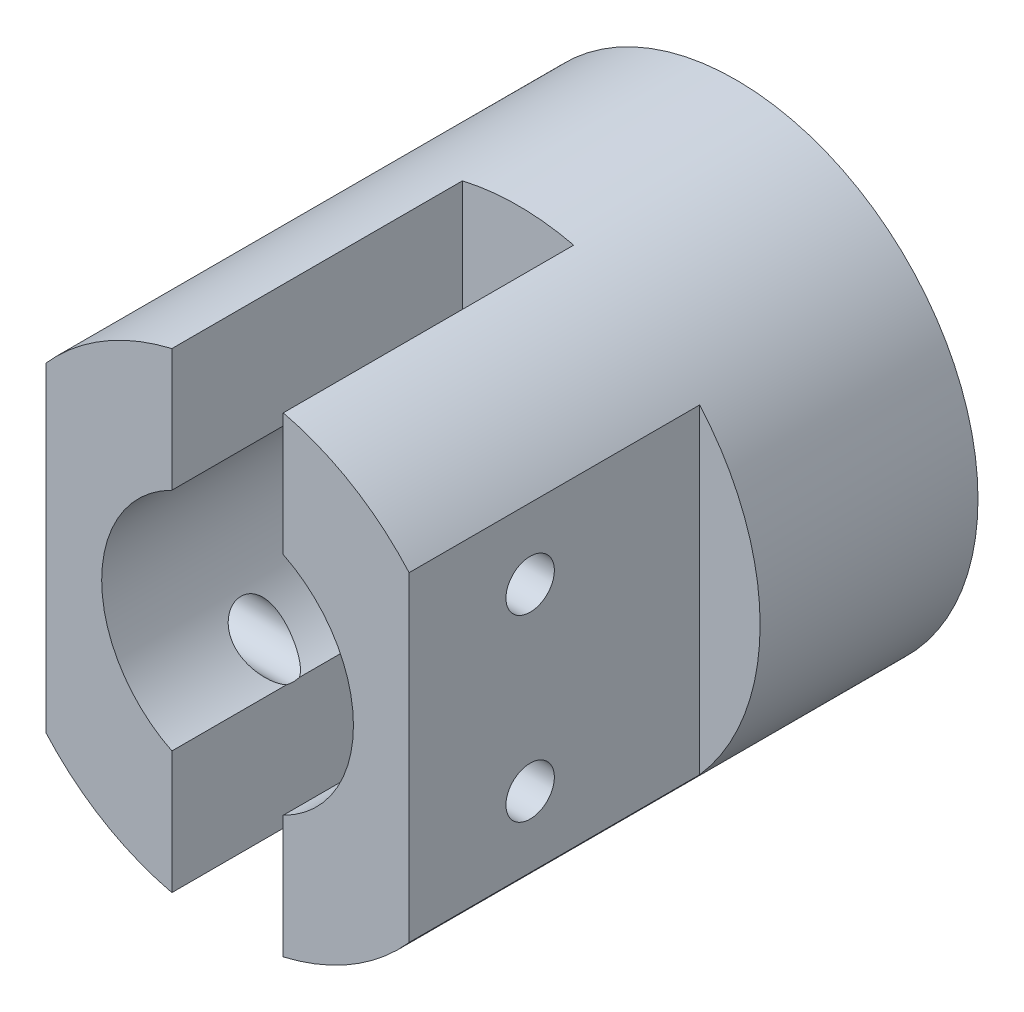
SolidWorks part; units mm, degrees
ref_plane "Front Plane" through (0, 0, 0) normal (0, 0, 1) x (1, 0, 0)
ref_plane "Top Plane" through (0, 0, 0) normal (0, 1, 0) x (1, 0, 0)
ref_plane "Right Plane" through (0, 0, 0) normal (1, 0, 0) x (0, 0, -1)
other "Configuration Table"
sketch "Sketch2" plane through (0, 0, 0) normal (0, 0, 1) x (1, 0, 0)
  circle A0 centre (0, 0) radius 5
  dimension "D1" = 10
extrude "Boss-Extrude1" add sketch "Sketch2" along normal blind 10.5
sketch "Sketch3" plane through (0, 0, 0) normal (0, 0, -1) x (-1, 0, 0)
  circle A0 centre (0, 0) radius 2.5
  dimension "D1" = 5
extrude "Cut-Extrude1" cut sketch "Sketch3" against normal blind 3.5
sketch "Sketch4" plane through (0, 0, 3.5) normal (0, 0, -1) x (-1, 0, 0)
  circle A0 centre (0, 0) radius 1
  dimension "D1" = 2
extrude "Cut-Extrude2" cut sketch "Sketch4" against normal through all
ref_plane "Plane1" through (0, 5, 0) normal (0, 1, 0) x (1, 0, 0)
sketch "Sketch5" plane through (0, 5, 0) normal (0, 1, 0) x (1, 0, 0)
  line L0 (-5, 0) -> (-5, -10.5) construction
  line L1 (-5, -4.5) -> (-3.75, -4.5)
  line L2 (-5, -4.5) -> (-5, -10.5)
  line L3 (-5, -10.5) -> (-3.75, -10.5)
  line L4 (-3.75, -4.5) -> (-3.75, -10.5)
  line L5 (-5, -10.5) -> (5, -10.5) construction
  line L6 (0, 0) -> (0, -11.4415) construction
  line L7 (5, -10.5) -> (3.75, -10.5)
  line L8 (5, -4.5) -> (5, -10.5)
  line L9 (5, -4.5) -> (3.75, -4.5)
  line L10 (3.75, -4.5) -> (3.75, -10.5)
  dimension "D1" = 6
  dimension "D2" = 1.25
extrude "Cut-Extrude3" cut sketch "Sketch5" against normal through all
sketch "Sketch6" plane through (0, 5, 0) normal (0, 1, 0) x (1, 0, 0)
  line L0 (-3.75, -10.5) -> (3.75, -10.5) construction
  line L1 (-1.15, -10.5) -> (1.15, -10.5)
  line L2 (-1.15, -10.5) -> (-1.15, -4.5)
  line L3 (-1.15, -4.5) -> (1.15, -4.5)
  line L4 (1.15, -10.5) -> (1.15, -4.5)
  line L6 (0, 0) -> (0, -10.8698) construction
  dimension "D1" = 6
  dimension "D2" = 2.3
  dimension "D3" = 1.15
extrude "Cut-Extrude4" cut sketch "Sketch6" against normal through all
sketch "Sketch7" plane through (0, 0, 10.5) normal (0, 0, 1) x (1, 0, 0)
  circle A1 centre (0, 0) radius 2.6
  dimension "D1" = 5.2
extrude "Cut-Extrude5" cut sketch "Sketch7" against normal up to surface (6 mm away) up to face at (-1, 0, 4.5)
sketch "Sketch8" plane through (-3.75, 0, 0) normal (-1, 0, 0) x (0, 0, 1)
  line L0 (0, 0) -> (13.184, 0) construction
  line L1 (10.5, -3.3072) -> (10.5, 3.3072) construction
  circle A0 centre (8, 1.85) radius 0.5
  circle A1 centre (8, -1.85) radius 0.5
  dimension "D1" = 1
  dimension "D2" = 1
  dimension "D3" = 1.85
  dimension "D4" = 1.85
  dimension "D5" = 2.5
  dimension "D6" = 2.5
extrude "Cut-Extrude6" cut sketch "Sketch8" against normal through all
